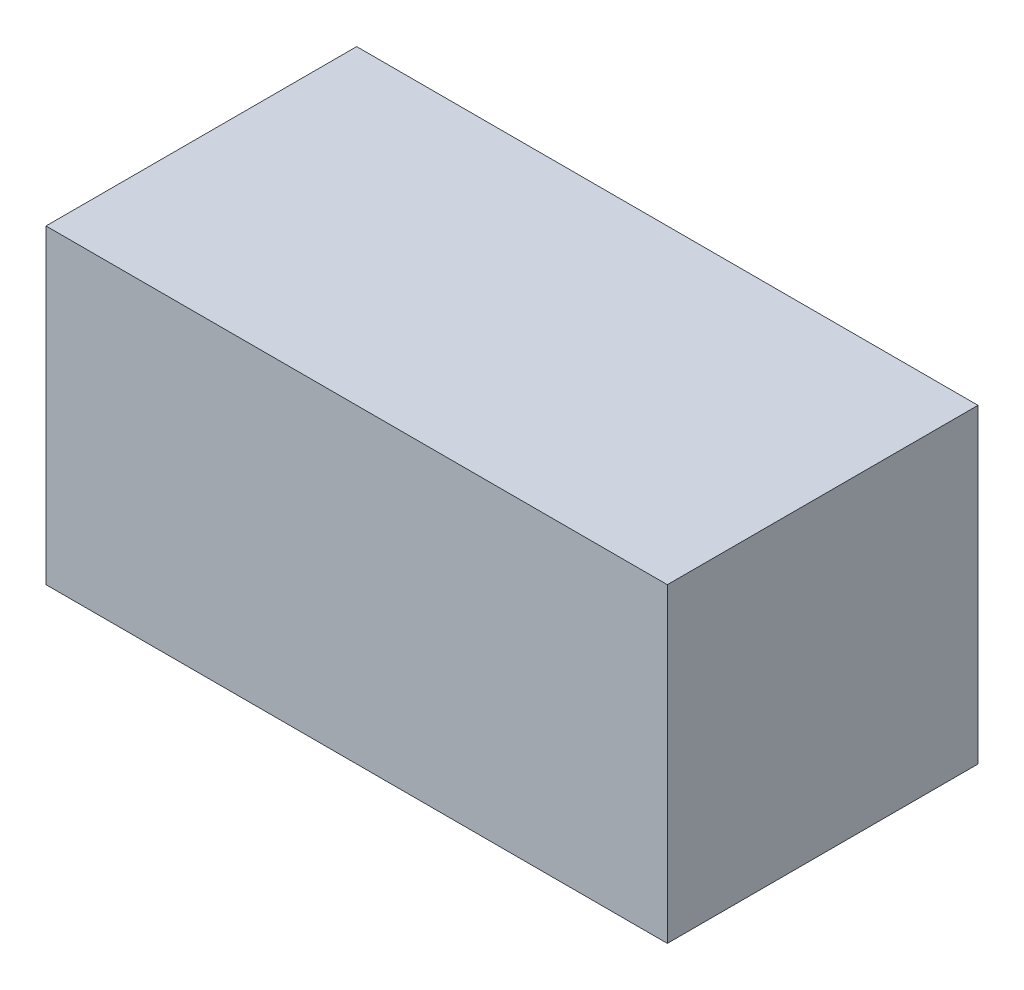
from build123d import *

# Parameters (mm, degrees)
SKETCH1_W           = 60
SKETCH1_H           = 30
BOSS_EXTRUDE1_DEPTH = 30


with BuildPart() as part:
    # Sketch1 → Boss-Extrude1 (new body)
    with BuildSketch(Plane.XY):
        with Locations((30, 15)):
            Rectangle(SKETCH1_W, SKETCH1_H)
    extrude(amount=BOSS_EXTRUDE1_DEPTH)


solid = part.part
